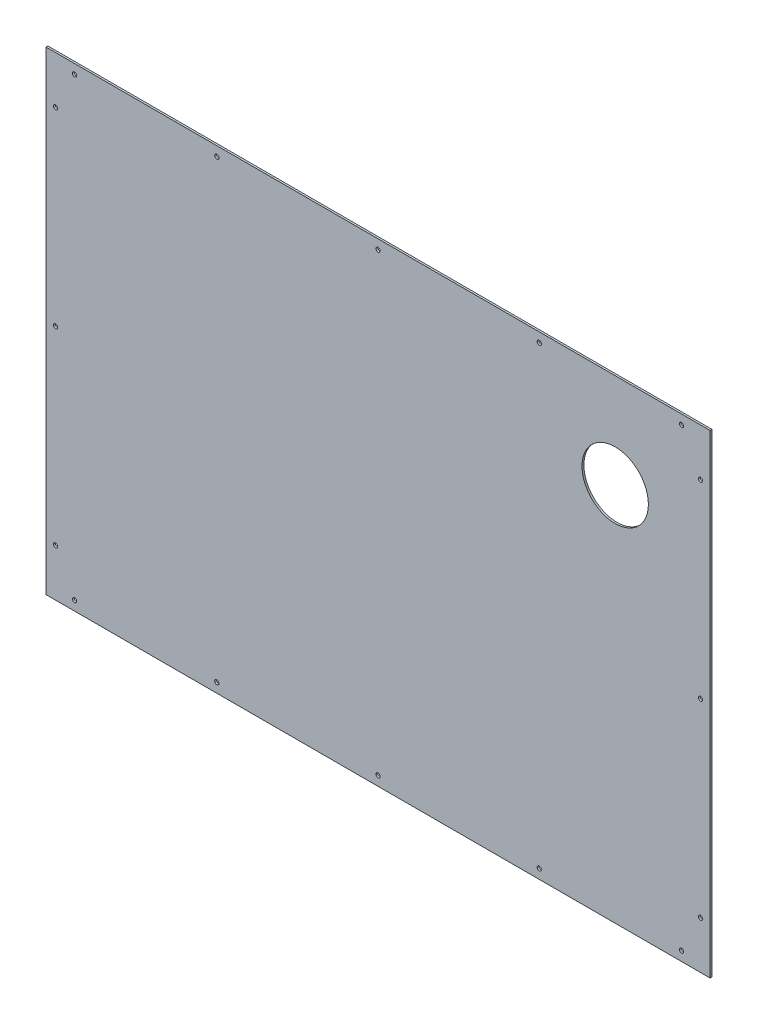
from build123d import *

# Parameters (mm, degrees)
SKETCH_1_W              = 700
SKETCH_1_H              = 500
EXTRUDE_1_DEPTH         = 2
HOLE_WIZARD_4_5_4_5_1_D = 4.5
SKETCH_4_R              = 35
CUT_EXTRUDE_1_DEPTH     = 10


with BuildPart() as part:
    # 草图1 → 凸台-拉伸1 (new body)
    with BuildSketch(Plane.XY):
        Rectangle(SKETCH_1_W, SKETCH_1_H)
    extrude(amount=EXTRUDE_1_DEPTH)

    # Ø4.5 (4.5) 直径孔1 (through all)
    with Locations(Plane.XY.offset(2)):
        with Locations((320, -240), (-340, 0), (0, -240), (340, 0), (0, 240), (-170, 240), (170, 240), (-170, -240), (170, -240), (-320, 240), (320, 240), (-340, 200), (-340, -200), (340, -200), (340, 200), (-320, -240)):
            Hole(HOLE_WIZARD_4_5_4_5_1_D / 2)

    # 草图4 → 切除-拉伸1 (cut)
    with BuildSketch(Plane.XY.offset(2)):
        with Locations((250, 150)):
            Circle(SKETCH_4_R)
    extrude(amount=-CUT_EXTRUDE_1_DEPTH, mode=Mode.SUBTRACT)


solid = part.part
